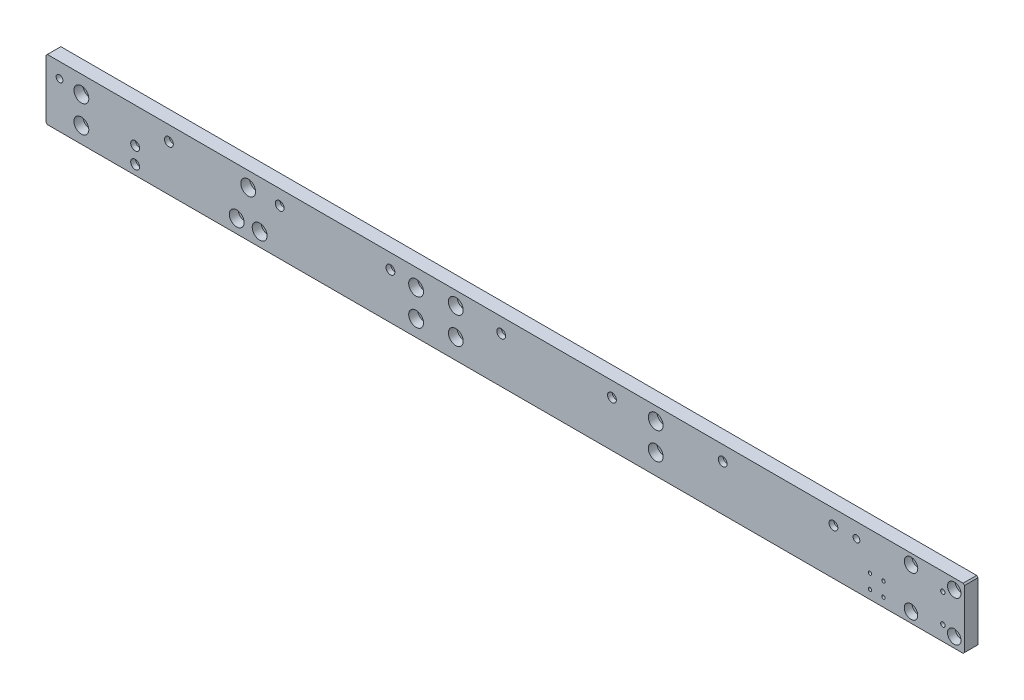
SolidWorks part; units mm, degrees
material "6061-T6 (SS)"
ref_plane "前视基准面" through (0, 0, 0) normal (0, 0, 1) x (1, 0, 0)
ref_plane "上视基准面" through (0, 0, 0) normal (0, 1, 0) x (1, 0, 0)
ref_plane "右视基准面" through (0, 0, 0) normal (1, 0, 0) x (0, 0, -1)
sketch "草图1" plane through (0, 0, 0) normal (0, 0, 1) x (1, 0, 0)
  line L1 (-400, 17) -> (310, 17)
  line L2 (-400, 17) -> (-400, -28)
  line L3 (-400, -28) -> (310, -28)
  line L4 (310, 17) -> (310, -28)
  dimension "D1" = 45
  dimension "D2" = 710
extrude "凸台-拉伸1" add sketch "草图1" against normal blind 10
hole_wizard "打孔尺寸根据六角头螺栓 C 级的类型2" positions "草图4" profile "草图3" counterbore size "M6" standard "Gb" end condition through all
sketch "草图4" plane through (0, 0, -10) normal (0, 0, -1) x (-1, 0, 0)
  line L1 (-310, -28) -> (-310, 17) construction
  point P3 (-213, 6)
  dimension "D1" = 97
sketch "草图3" plane through (213, 6, -10) normal (1, 0, 0) x (0, 1, 0)
  line L0 (0, 0) -> (0, 10)
  line L1 (0, 10) -> (3.25, 10)
  line L3 (3.25, 10) -> (3.25, 6.5)
  line L4 (3.25, 6.5) -> (5.5, 6.5)
  line L5 (5.5, 6.5) -> (5.5, 0)
  line L7 (5.5, 0) -> (0, 0)
  line L11 (0, -6.35) -> (0, 107.95) construction
  dimension "通孔孔直径" = 6.5
  dimension "通孔孔深度" = 10
  dimension "柱形沉头孔直径" = 11
  dimension "柱形沉头孔深度" = 6.5
pattern_linear "阵列(线性)1" count 7 spacing 82 along (-1, 0, 0) of "打孔尺寸根据六角头螺栓 C 级的类型2"
hole_wizard "打孔尺寸根据六角头螺栓 C 级的类型1" positions "草图6" profile "草图5" counterbore size "M6" standard "Gb" end condition through all
sketch "草图6" plane through (0, 0, 0) normal (0, 0, 1) x (1, 0, 0)
  line L0 (310, 17) -> (-400, 17) construction
  line L1 (-400, 17) -> (-400, -28) construction
  point P3 (-343.82, -16)
  point P8 (-343.82, 4)
  dimension "D1" = 13
  dimension "D2" = 20
  dimension "D3" = 56.18
sketch "草图5" plane through (-343.82, -16, 0) normal (1, 0, 0) x (0, -1, 0)
  line L0 (0, 0) -> (0, 10)
  line L1 (0, 10) -> (3.3, 10)
  line L3 (3.3, 10) -> (3.3, 6.6)
  line L4 (3.3, 6.6) -> (5.5, 6.6)
  line L5 (5.5, 6.6) -> (5.5, 0)
  line L7 (5.5, 0) -> (0, 0)
  line L11 (0, -6.35) -> (0, 107.95) construction
  dimension "通孔孔直径" = 6.6
  dimension "通孔孔深度" = 10
  dimension "柱形沉头孔直径" = 11
  dimension "柱形沉头孔深度" = 6.6
hole_wizard "打孔尺寸根据六角头螺栓 C 级的类型2" positions "草图8" profile "草图7" counterbore size "M6" standard "Gb" end condition through all
sketch "草图8" plane through (0, 0, 0) normal (0, 0, 1) x (1, 0, 0)
  line L0 (-400, 17) -> (-400, -28) construction
  line L1 (310, 17) -> (-400, 17) construction
  point P0 (-96, -16)
  point P3 (-96, 4)
  dimension "D1" = 304
  dimension "D2" = 13
  dimension "D3" = 20
sketch "草图7" plane through (-96, -16, 0) normal (1, 0, 0) x (0, -1, 0)
  line L0 (0, 0) -> (0, 10)
  line L1 (0, 10) -> (3.3, 10)
  line L3 (3.3, 10) -> (3.3, 6.6)
  line L4 (3.3, 6.6) -> (5.5, 6.6)
  line L5 (5.5, 6.6) -> (5.5, 0)
  line L7 (5.5, 0) -> (0, 0)
  line L11 (0, -6.35) -> (0, 107.95) construction
  dimension "通孔孔直径" = 6.6
  dimension "通孔孔深度" = 10
  dimension "柱形沉头孔直径" = 11
  dimension "柱形沉头孔深度" = 6.6
hole_wizard "打孔尺寸根据六角头螺栓 C 级的类型3" positions "草图10" profile "草图9" counterbore size "M6" standard "Gb" end condition through all
sketch "草图10" plane through (0, 0, 0) normal (0, 0, 1) x (1, 0, 0)
  line L4 (-400, -28) -> (310, -28) construction
  line L5 (-400, 17) -> (-400, -28) construction
  point P0 (-228.82, -18)
  point P2 (-211.82, -18)
  point P4 (-220.32, 6)
  dimension "D1" = 171.18
  dimension "D2" = 17
  dimension "D3" = 10
  dimension "D4" = 24
  dimension "D5" = 8.5
sketch "草图9" plane through (-228.82, -18, 0) normal (1, 0, 0) x (0, -1, 0)
  line L0 (0, 0) -> (0, 10)
  line L1 (0, 10) -> (3.25, 10)
  line L3 (3.25, 10) -> (3.25, 6.5)
  line L4 (3.25, 6.5) -> (5.5, 6.5)
  line L5 (5.5, 6.5) -> (5.5, 0)
  line L7 (5.5, 0) -> (0, 0)
  line L11 (0, -6.35) -> (0, 107.95) construction
  dimension "通孔孔直径" = 6.5
  dimension "通孔孔深度" = 10
  dimension "柱形沉头孔直径" = 11
  dimension "柱形沉头孔深度" = 6.5
hole_wizard "M6 六角凹头螺钉的柱形沉头孔1" positions "草图12" profile "草图11" counterbore size "M6" standard "Iso" end condition through all
sketch "草图12" plane through (0, 0, -10) normal (0, 0, -1) x (-1, 0, 0)
  line L1 (400, -28) -> (-310, -28) construction
  line L2 (400, 17) -> (400, -28) construction
  point P0 (304, -21)
  point P3 (304, -9)
  dimension "D1" = 7
  dimension "D2" = 12
  dimension "D3" = 96
sketch "草图11" plane through (-304, -21, -10) normal (1, 0, 0) x (0, 1, 0)
  line L0 (0, 0) -> (0, 10)
  line L1 (0, 10) -> (3.3, 10)
  line L3 (3.3, 10) -> (3.3, 6.4)
  line L4 (3.3, 6.4) -> (5.5, 6.4)
  line L5 (5.5, 6.4) -> (5.5, 0)
  line L7 (5.5, 0) -> (0, 0)
  line L11 (0, -6.35) -> (0, 107.95) construction
  dimension "通孔孔直径" = 6.6
  dimension "通孔孔深度" = 10
  dimension "柱形沉头孔直径" = 11
  dimension "柱形沉头孔深度" = 6.4
hole_wizard "M6 六角凹头螺钉的柱形沉头孔2" positions "草图14" profile "草图13" counterbore size "M6" standard "Iso" end condition through all
sketch "草图14" plane through (0, 0, 0) normal (0, 0, 1) x (1, 0, 0)
  line L0 (310, 17) -> (-400, 17) construction
  point P0 (81.4, 7)
  point P3 (81.4, -13)
  point P8 (-66.6, 7)
  point P11 (-66.6, -13)
  dimension "D1" = 10
  dimension "D2" = 20
  dimension "D3" = 10
  dimension "D4" = 20
  dimension "D5" = 148
sketch "草图13" plane through (81.4, 7, 0) normal (1, 0, 0) x (0, -1, 0)
  line L0 (0, 0) -> (0, 10)
  line L1 (0, 10) -> (3.3, 10)
  line L3 (3.3, 10) -> (3.3, 6.4)
  line L4 (3.3, 6.4) -> (5.5, 6.4)
  line L5 (5.5, 6.4) -> (5.5, 0)
  line L7 (5.5, 0) -> (0, 0)
  line L11 (0, -6.35) -> (0, 107.95) construction
  dimension "通孔孔直径" = 6.6
  dimension "通孔孔深度" = 10
  dimension "柱形沉头孔直径" = 11
  dimension "柱形沉头孔深度" = 6.4
chamfer "倒角1" distance 1 angle 45 4 edges at (310, -28, -5) (310, 17, -5) (-400, -28, -5) (-400, 17, -5)
hole_wizard "Ø5.0 (5) 直径孔1" positions "草图16" profile "草图15" hole size "Ø5.0" standard "Ansi Metric"
sketch "草图16" plane through (0, 0, 0) normal (0, 0, 1) x (1, 0, 0)
  line L0 (-399, -28) -> (309, -28) construction
  line L1 (-400, 16) -> (-400, -27) construction
  line L2 (310, -27) -> (310, 16) construction
  point P0 (230, 6)
  point P2 (-360, 6)
  dimension "D1" = 34
  dimension "D2" = 40
  dimension "D3" = 80
sketch "草图15" plane through (230, 6, 0) normal (1, 0, 0) x (0, -1, 0)
  line L0 (0, 0) -> (0, 17.0534)
  line L1 (0, 17.0534) -> (2.5, 15.61)
  line L2 (2.5, 15.61) -> (2.5, 0)
  line L5 (2.5, 0) -> (0, 0)
  line L10 (0, 17.0534) -> (-2.5, 15.61) construction
  line L11 (0, -6.35) -> (0, 107.95) construction
  dimension "孔直径" = 5
  dimension "孔深度" = 15.61
  dimension "导头角度" = 120
hole_wizard "打孔尺寸根据内六角圆柱头螺钉的类型1" positions "草图18" profile "草图17" counterbore size "M5" standard "Gb" end condition through all
sketch "草图18" plane through (0, 0, 0) normal (0, 0, 1) x (1, 0, 0)
  line L0 (310, -27) -> (310, 16) construction
  line L1 (309, 17) -> (-399, 17) construction
  point P0 (270.4, 9.5)
  point P3 (302.4, 9.5)
  point P6 (270.4, -20.5)
  point P9 (302.4, -20.5)
  dimension "D1" = 7.6
  dimension "D2" = 7.5
  dimension "D3" = 30
  dimension "D4" = 32
sketch "草图17" plane through (270.4, 9.5, 0) normal (1, 0, 0) x (0, -1, 0)
  line L0 (0, 0) -> (0, 10)
  line L1 (0, 10) -> (2.65, 10)
  line L3 (2.65, 10) -> (2.65, 5.7)
  line L4 (2.65, 5.7) -> (5, 5.7)
  line L5 (5, 5.7) -> (5, 0)
  line L7 (5, 0) -> (0, 0)
  line L11 (0, -6.35) -> (0, 107.95) construction
  dimension "通孔孔直径" = 5.3
  dimension "通孔孔深度" = 10
  dimension "柱形沉头孔直径" = 10
  dimension "柱形沉头孔深度" = 5.7
hole_wizard "M4 螺纹孔1" positions "草图20" profile "草图19" tap size "M4" standard "Iso"
sketch "草图20" plane through (0, 0, 0) normal (0, 0, 1) x (1, 0, 0)
  line L0 (310, -27) -> (310, 16) construction
  line L1 (-399, -28) -> (309, -28) construction
  point P0 (294, 4)
  point P2 (294, -17)
  dimension "D1" = 16
  dimension "D2" = 11
  dimension "D3" = 21
sketch "草图19" plane through (294, 4, 0) normal (1, 0, 0) x (0, -1, 0)
  line L0 (0, 0) -> (0, 11.0914)
  line L1 (0, 11.0914) -> (1.65, 10.1)
  line L2 (1.65, 10.1) -> (1.65, 0)
  line L5 (1.65, 0) -> (0, 0)
  line L10 (0, 11.0914) -> (-1.65, 10.1) construction
  line L11 (0, -6.35) -> (0, 107.95) construction
  dimension "螺纹孔钻头直径" = 3.3
  dimension "螺纹孔钻头深度" = 10.1
  dimension "导头角度" = 118
cosmetic thread "孔螺蚊线1" parameters "D1"=8, "D2"=4
cosmetic thread "孔螺蚊线2" parameters "D1"=8, "D2"=4
sketch "草图21" plane through (0, 0, 0) normal (0, 0, 1) x (1, 0, 0)
  line L0 (-370, 48.2163) -> (-370, -32.8711)
extrude "切除-拉伸1" cut sketch "草图21" against normal through all and the other way through all flip side to cut
chamfer "倒角2" distance 1 angle 45 2 edges at (-370, 17, -5) (-370, -28, -5)
hole_wizard "M3 螺纹孔1" positions "草图23" profile "草图22" tap size "M3" standard "Iso"
sketch "草图23" plane through (0, 0, 0) normal (0, 0, 1) x (1, 0, 0)
  line L0 (310, -27) -> (310, 16) construction
  line L1 (-369, -28) -> (309, -28) construction
  point P0 (240, -21.5)
  point P3 (240, -11.1)
  point P6 (250, -11.1)
  point P9 (250, -21.5)
  dimension "D1" = 10
  dimension "D2" = 10.4
  dimension "D3" = 60
  dimension "D4" = 6.5
sketch "草图22" plane through (240, -21.5, 0) normal (1, 0, 0) x (0, -1, 0)
  line L0 (0, 0) -> (0, 8.2511)
  line L1 (0, 8.2511) -> (1.25, 7.5)
  line L2 (1.25, 7.5) -> (1.25, 0)
  line L5 (1.25, 0) -> (0, 0)
  line L10 (0, 8.2511) -> (-1.25, 7.5) construction
  line L11 (0, -6.35) -> (0, 107.95) construction
  dimension "螺纹孔钻头直径" = 2.5
  dimension "螺纹孔钻头深度" = 7.5
  dimension "导头角度" = 118
cosmetic thread "孔螺蚊线3" parameters "D1"=6, "D2"=3
cosmetic thread "孔螺蚊线4" parameters "D1"=6, "D2"=3
cosmetic thread "孔螺蚊线5" parameters "D1"=6, "D2"=3
cosmetic thread "孔螺蚊线6" parameters "D1"=6, "D2"=3
